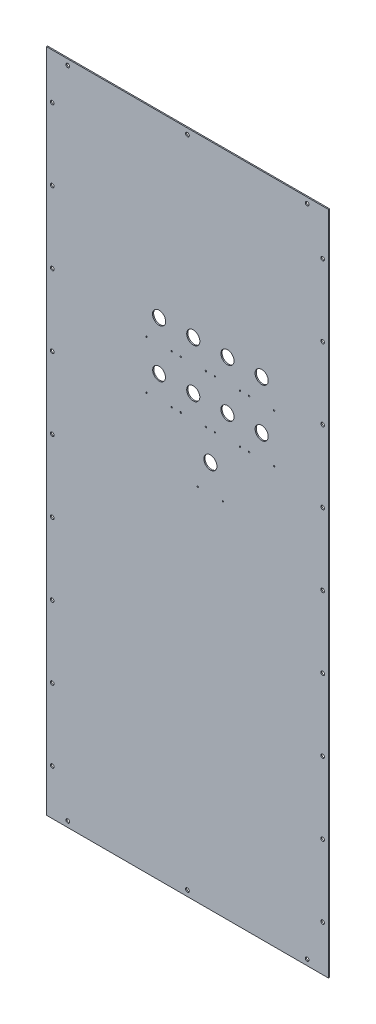
SolidWorks part; units mm, degrees
material "304"
ref_plane "前视基准面" through (0, 0, 0) normal (0, 0, 1) x (1, 0, 0)
ref_plane "上视基准面" through (0, 0, 0) normal (0, 1, 0) x (1, 0, 0)
ref_plane "右视基准面" through (0, 0, 0) normal (1, 0, 0) x (0, 0, -1)
sketch "草图1" plane through (0, 0, 0) normal (0, 0, 1) x (1, 0, 0)
  line L0 (0, 0) -> (451.2544, 0) construction
  line L1 (-247.25, 584) -> (247.25, 584)
  line L2 (-247.25, 584) -> (-247.25, -584)
  line L3 (-247.25, -584) -> (247.25, -584)
  line L4 (247.25, 584) -> (247.25, -584)
  line L5 (-247.25, 584) -> (247.25, -584) construction
  line L6 (-247.25, -584) -> (247.25, 584) construction
  line L7 (0, 0) -> (0, 412.8629) construction
  circle A0 centre (-237.25, 0) radius 3.25
  circle A1 centre (-237.25, -126) radius 3.25
  circle A2 centre (-237.25, -252) radius 3.25
  circle A3 centre (-237.25, -378) radius 3.25
  circle A4 centre (-237.25, -504) radius 3.25
  circle A34 centre (0, -574) radius 3.25
  circle A35 centre (0, 574) radius 3.25
  circle A36 centre (-237.25, 504) radius 3.25
  circle A37 centre (-237.25, 378) radius 3.25
  circle A38 centre (-237.25, 252) radius 3.25
  circle A39 centre (-237.25, 126) radius 3.25
  circle A40 centre (237.25, 126) radius 3.25
  circle A41 centre (237.25, 252) radius 3.25
  circle A42 centre (237.25, 378) radius 3.25
  circle A43 centre (237.25, 504) radius 3.25
  circle A44 centre (237.25, -504) radius 3.25
  circle A45 centre (237.25, -378) radius 3.25
  circle A46 centre (237.25, -252) radius 3.25
  circle A47 centre (237.25, -126) radius 3.25
  circle A48 centre (237.25, 0) radius 3.25
  circle A49 centre (-210, 574) radius 3.25
  circle A50 centre (210, 574) radius 3.25
  circle A51 centre (210, -574) radius 3.25
  circle A52 centre (-210, -574) radius 3.25
  point P0 (0, 0)
  dimension "D3" = 6.5
  dimension "D8" = 420
  dimension "D1" = 494.5
  dimension "D2" = 1168
  dimension "D4" = 10
  dimension "D6" = 10
  dimension "D7" = 80
  dimension "D5" = 5
extrude "凸台-拉伸1" add sketch "草图1" along normal blind 2
sketch "草图2" plane through (0, -584, 0) normal (0, -1, 0) x (1, 0, 0)
  line L0 (-247.25, 2) -> (247.25, 2) construction
  line L1 (247.25, 0) -> (244.75, 0)
  line L2 (247.25, 0) -> (247.25, 2)
  line L3 (247.25, 2) -> (244.75, 2)
  line L4 (244.75, 0) -> (244.75, 2)
  dimension "D1" = 2.5
sketch "草图3" plane through (0, 0, 0) normal (0, 0, -1) x (-1, 0, 0)
  circle A2 centre (-48.25, 145.8325) radius 1.15
  circle A4 centre (-10.25, 185.8325) radius 11.5
  circle A6 centre (-32.25, 145.8325) radius 1.15
  circle A8 centre (11.75, 145.8325) radius 1.15
  circle A10 centre (27.75, 145.8325) radius 1.15
  circle A12 centre (71.75, 145.8325) radius 1.15
  circle A14 centre (49.75, 270.8325) radius 11.5
  circle A16 centre (27.75, 230.8325) radius 1.15
  circle A18 centre (71.75, 230.8325) radius 1.15
  circle A20 centre (-130.25, 185.8325) radius 11.5
  circle A22 centre (-152.25, 145.8325) radius 1.15
  circle A24 centre (-108.25, 145.8325) radius 1.15
  circle A26 centre (-70.25, 185.8325) radius 11.5
  circle A28 centre (-92.25, 145.8325) radius 1.15
  circle A30 centre (-152.25, 230.8325) radius 1.15
  circle A32 centre (-108.25, 230.8325) radius 1.15
  circle A34 centre (-70.25, 270.8325) radius 11.5
  circle A36 centre (-92.25, 230.8325) radius 1.15
  circle A38 centre (-48.25, 230.8325) radius 1.15
  circle A40 centre (-10.25, 270.8325) radius 11.5
  circle A42 centre (-32.25, 230.8325) radius 1.15
  circle A44 centre (11.75, 230.8325) radius 1.15
  circle A46 centre (-40.25, 95.8325) radius 11.5
  circle A48 centre (-62.25, 47.8325) radius 1.15
  circle A50 centre (-18.25, 47.8325) radius 1.15
  circle A52 centre (-130.25, 270.8325) radius 11.5
  circle A54 centre (49.75, 185.8325) radius 11.25
  point P0 (0, 0)
extrude "切除-拉伸2" cut sketch "草图3" against normal blind 10
